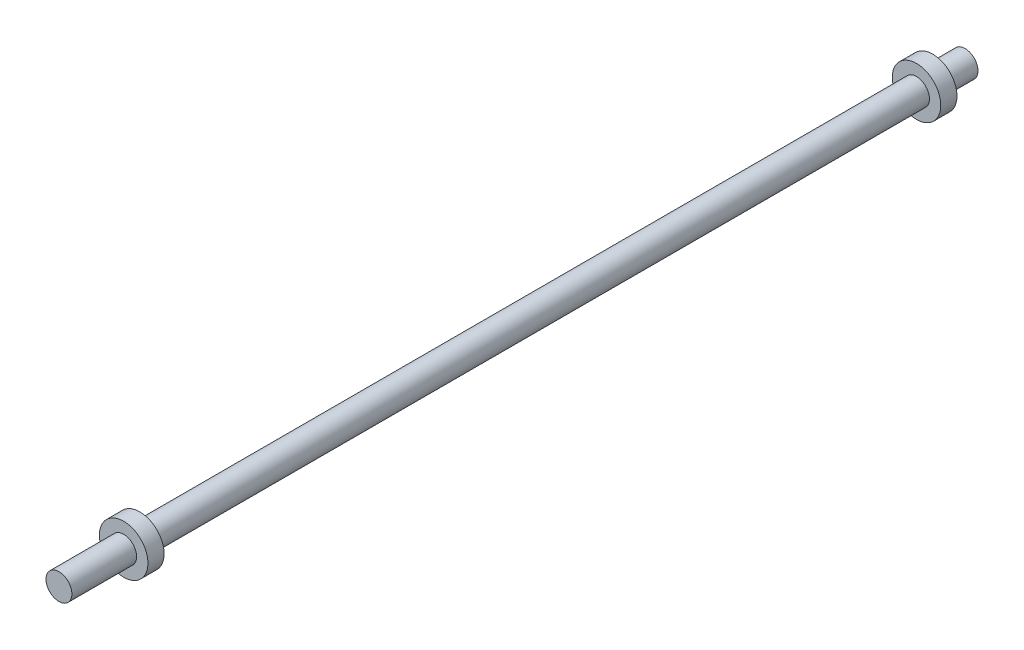
from build123d import *

# Parameters (mm, degrees)
SKETCH_1_R      = 4
EXTRUDE_1_DEPTH = 140
EXTRUDE_START   = -20
SKETCH_2_R      = 7.5
EXTRUDE_2_DEPTH = 5
EXTRUDE_START_2 = -15
SKETCH_3_R      = 7.5
EXTRUDE_3_DEPTH = 5


with BuildPart() as part:
    # 草图1 → 凸台-拉伸1 (new, symmetric)
    with BuildSketch(Plane.XY):
        Circle(SKETCH_1_R)
    extrude(amount=EXTRUDE_1_DEPTH, both=True)

    # 草图2 → 凸台-拉伸2 (add)
    with BuildSketch(Plane.XY.offset(140).offset(EXTRUDE_START)):
        Circle(SKETCH_2_R)
    extrude(amount=-EXTRUDE_2_DEPTH)

    # 草图3 → 凸台-拉伸3 (add)
    with BuildSketch(Plane(origin=(0, 0, -140), x_dir=(-1, 0, 0), z_dir=(0, 0, -1)).offset(EXTRUDE_START_2)):
        with Locations(Location((0, 0, 0), (0, 0, 180))):
            Circle(SKETCH_3_R)
    extrude(amount=EXTRUDE_3_DEPTH)


solid = part.part
